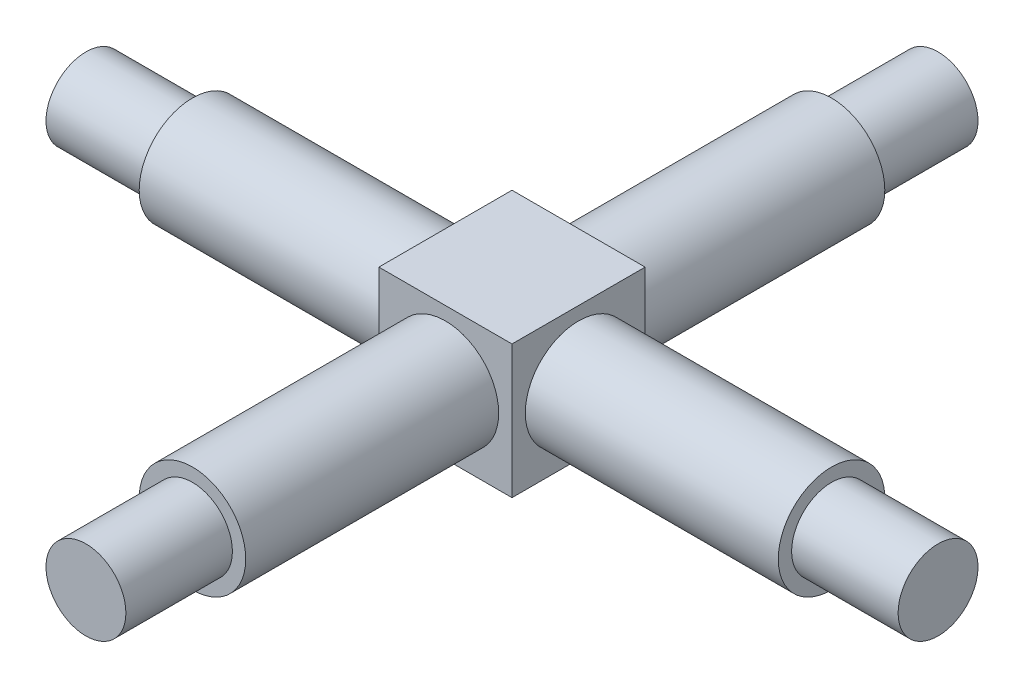
SolidWorks part; units mm, degrees
material "S45C"
ref_plane "Front Plane" through (0, 0, 0) normal (0, 0, 1) x (1, 0, 0)
ref_plane "Top Plane" through (0, 0, 0) normal (0, 1, 0) x (1, 0, 0)
ref_plane "Right Plane" through (0, 0, 0) normal (1, 0, 0) x (0, 0, -1)
other "Configuration Table"
sketch "Sketch1" plane through (0, 0, 0) normal (0, 0, 1) x (1, 0, 0)
  line L0 (-30.6936, 30.799) -> (-25.6936, 30.799)
  line L1 (-25.6936, 30.799) -> (-25.6936, 25.799)
  line L2 (-25.6936, 25.799) -> (-30.6936, 25.799)
  line L3 (-30.6936, 25.799) -> (-30.6936, 30.799)
extrude "Boss-Extrude1" add sketch "Sketch1" along normal blind 5
sketch "Sketch2" plane through (0, 0, 5) normal (0, 0, 1) x (1, 0, 0)
  circle A0 centre (-28.1936, 28.299) radius 2
  dimension "D1" = 4
extrude "Boss-Extrude2" add sketch "Sketch2" along normal blind 13.5
sketch "Sketch3" plane through (-25.6936, 0, 0) normal (1, 0, 0) x (0, 0, -1)
  circle A0 centre (-2.5, 28.299) radius 2
  dimension "D1" = 4
extrude "Boss-Extrude3" add sketch "Sketch3" along normal blind 13.5
ref_plane "Plane1" through (0, 0, 2.5) normal (0, 0, -1) x (-1, 0, 0)
mirror "Mirror1" about plane through (0, 0, 2.5) normal (0, 0, -1) of "Boss-Extrude2"
ref_plane "Plane2" through (-28.1936, 0, 0) normal (1, 0, 0) x (0, 0, -1)
mirror "Mirror2" about plane through (-28.1936, 0, 0) normal (1, 0, 0) of "Boss-Extrude3"
sketch "Sketch4" plane through (0, 0, 18.5) normal (0, 0, 1) x (1, 0, 0)
  circle A0 centre (-28.1936, 28.299) radius 1.5
  circle A1 centre (-28.1936, 28.299) radius 2
  dimension "D1" = 3
extrude "Cut-Extrude1" cut sketch "Sketch4" against normal blind 4
mirror "Mirror3" about plane through (0, 0, 2.5) normal (0, 0, -1) of "Cut-Extrude1"
sketch "Sketch5" plane through (-44.1936, 0, 0) normal (-1, 0, 0) x (0, 0, 1)
  circle A0 centre (2.5, 28.299) radius 2
  circle A1 centre (2.5, 28.299) radius 1.5
  dimension "D1" = 4
  dimension "D2" = 3
extrude "Cut-Extrude2" cut sketch "Sketch5" against normal blind 4
mirror "Mirror4" about plane through (-28.1936, 0, 0) normal (1, 0, 0) of "Cut-Extrude2"
